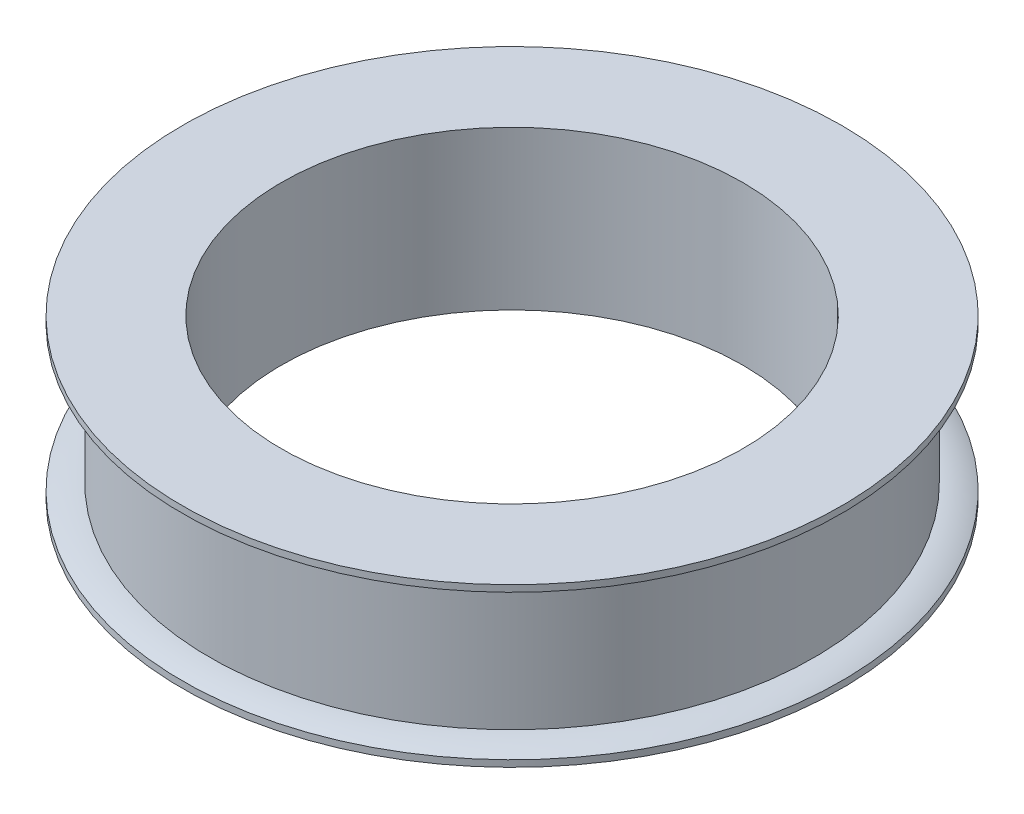
SolidWorks part; units mm, degrees
material "7075-T6"
ref_plane "Front Plane" through (0, 0, 0) normal (0, 0, 1) x (1, 0, 0)
ref_plane "Top Plane" through (0, 0, 0) normal (0, 1, 0) x (1, 0, 0)
ref_plane "Right Plane" through (0, 0, 0) normal (1, 0, 0) x (0, 0, -1)
sketch "Sketch1" plane through (0, 0, 0) normal (0, 0, 1) x (1, 0, 0)
  line L0 (17.5, 0) -> (22.92, 0) construction
  line L1 (22.92, -5) -> (22.92, 5)
  line L2 (22.92, 5) -> (20, 5)
  line L3 (20, 5) -> (20, 6)
  line L4 (20, 6) -> (17.5, 6)
  line L5 (17.5, 6) -> (17.5, -6)
  line L6 (0, 0) -> (0, 19.2388) construction
  line L7 (20, -6) -> (17.5, -6)
  line L8 (20, -5) -> (20, -6)
  line L9 (22.92, -5) -> (20, -5)
  dimension "D1" = 35
  dimension "D2" = 45.84
  dimension "D3" = 40
  dimension "D4" = 10
  dimension "D5" = 12
revolve "Revolve1" add sketch "Sketch1" angle 360 about L6
sketch "Sketch2" plane through (0, 0, 0) normal (0, 0, 1) x (1, 0, 0)
  line L0 (22.92, 0) -> (30.41, 0) construction
  line L1 (20, 5) -> (22.92, 5)
  line L2 (20, 5) -> (20, 6)
  line L3 (20, 6) -> (25, 6)
  line L4 (25, 5.5) -> (25, 6)
  line L5 (22.92, -5) -> (22.92, 5) construction
  line L6 (20, 6) -> (-20, 6) construction
  line L7 (0, 0) -> (0, 7.8829) construction
  line L12 (25, -5.5) -> (25, -6)
  line L13 (20, -6) -> (25, -6)
  line L14 (20, -5) -> (20, -6)
  line L15 (20, -5) -> (22.92, -5)
  arc A0 (22.92, 5) -> (25, 5.5) centre (22.8184, 9.999) ccw
  arc A1 (22.92, -5) -> (25, -5.5) centre (22.8184, -9.999) cw
  dimension "D3" = 5
  dimension "D1" = 50
  dimension "D2" = 0.5
revolve "Revolve2" add sketch "Sketch2" angle 360 about L7
